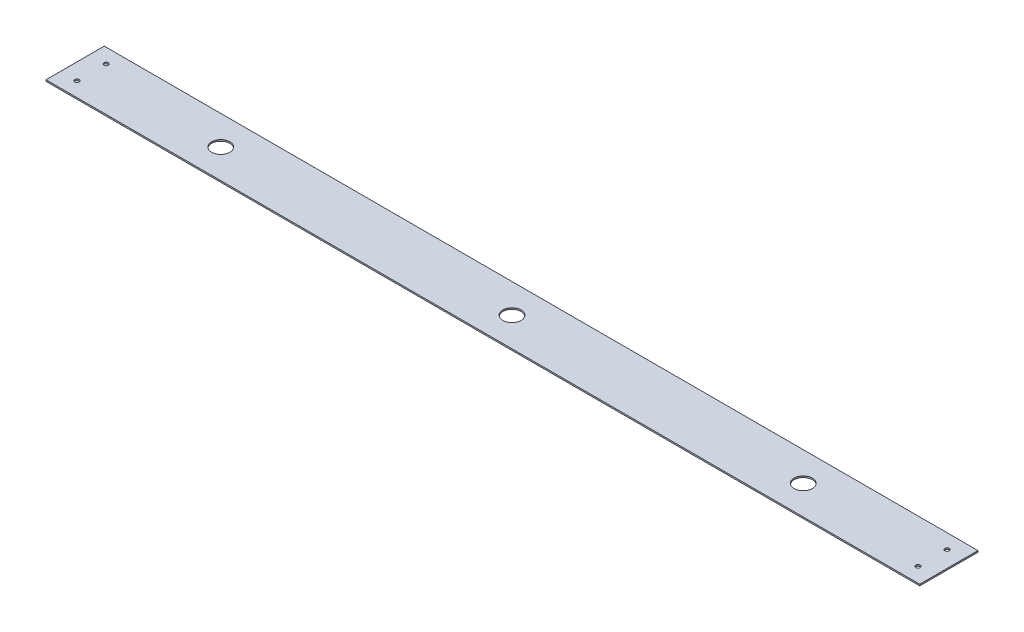
from build123d import *

# Parameters (mm, degrees)
SKETCH1_W           = 1200
SKETCH1_H           = 80
SKETCH1_R           = 12.5
SKETCH1_R_2         = 3
BOSS_EXTRUDE1_DEPTH = 2


with BuildPart() as part:
    # Sketch1 → Boss-Extrude1 (new body)
    with BuildSketch(Plane(origin=(0, 0, 0), x_dir=(1, 0, 0), z_dir=(0, 1, 0))):
        Rectangle(SKETCH1_W, SKETCH1_H)
        with Locations(Location((-400, 0, 0), (0, 0, 270))):
            Circle(SKETCH1_R, mode=Mode.SUBTRACT)
        with Locations(Location((400, 0, 0), (0, 0, 270))):
            Circle(SKETCH1_R, mode=Mode.SUBTRACT)
        with Locations(Location((-577.5, 20, 0), (0, 0, 270))):
            Circle(SKETCH1_R_2, mode=Mode.SUBTRACT)
        with Locations(Location((577.5, 20, 0), (0, 0, 270))):
            Circle(SKETCH1_R_2, mode=Mode.SUBTRACT)
        with Locations(Location((-577.5, -20, 0), (0, 0, 270))):
            Circle(SKETCH1_R_2, mode=Mode.SUBTRACT)
        with Locations(Location((577.5, -20, 0), (0, 0, 270))):
            Circle(SKETCH1_R_2, mode=Mode.SUBTRACT)
        with Locations(Location((0, 0, 0), (0, 0, 270))):
            Circle(SKETCH1_R, mode=Mode.SUBTRACT)
    extrude(amount=BOSS_EXTRUDE1_DEPTH)


solid = part.part
